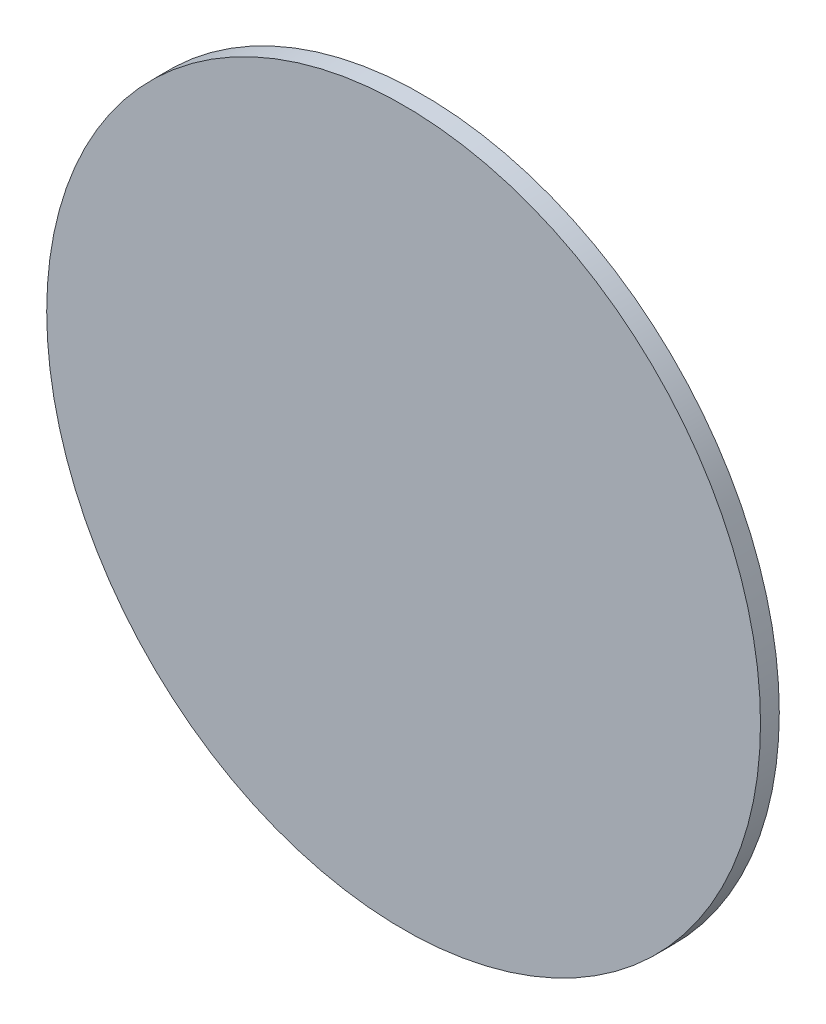
from build123d import *

# Parameters (mm, degrees)
SKETCH1_R           = 380
BOSS_EXTRUDE1_DEPTH = 20


with BuildPart() as part:
    # Sketch1 → Boss-Extrude1 (new body)
    with BuildSketch(Plane.XY):
        Circle(SKETCH1_R)
    extrude(amount=BOSS_EXTRUDE1_DEPTH)


solid = part.part
